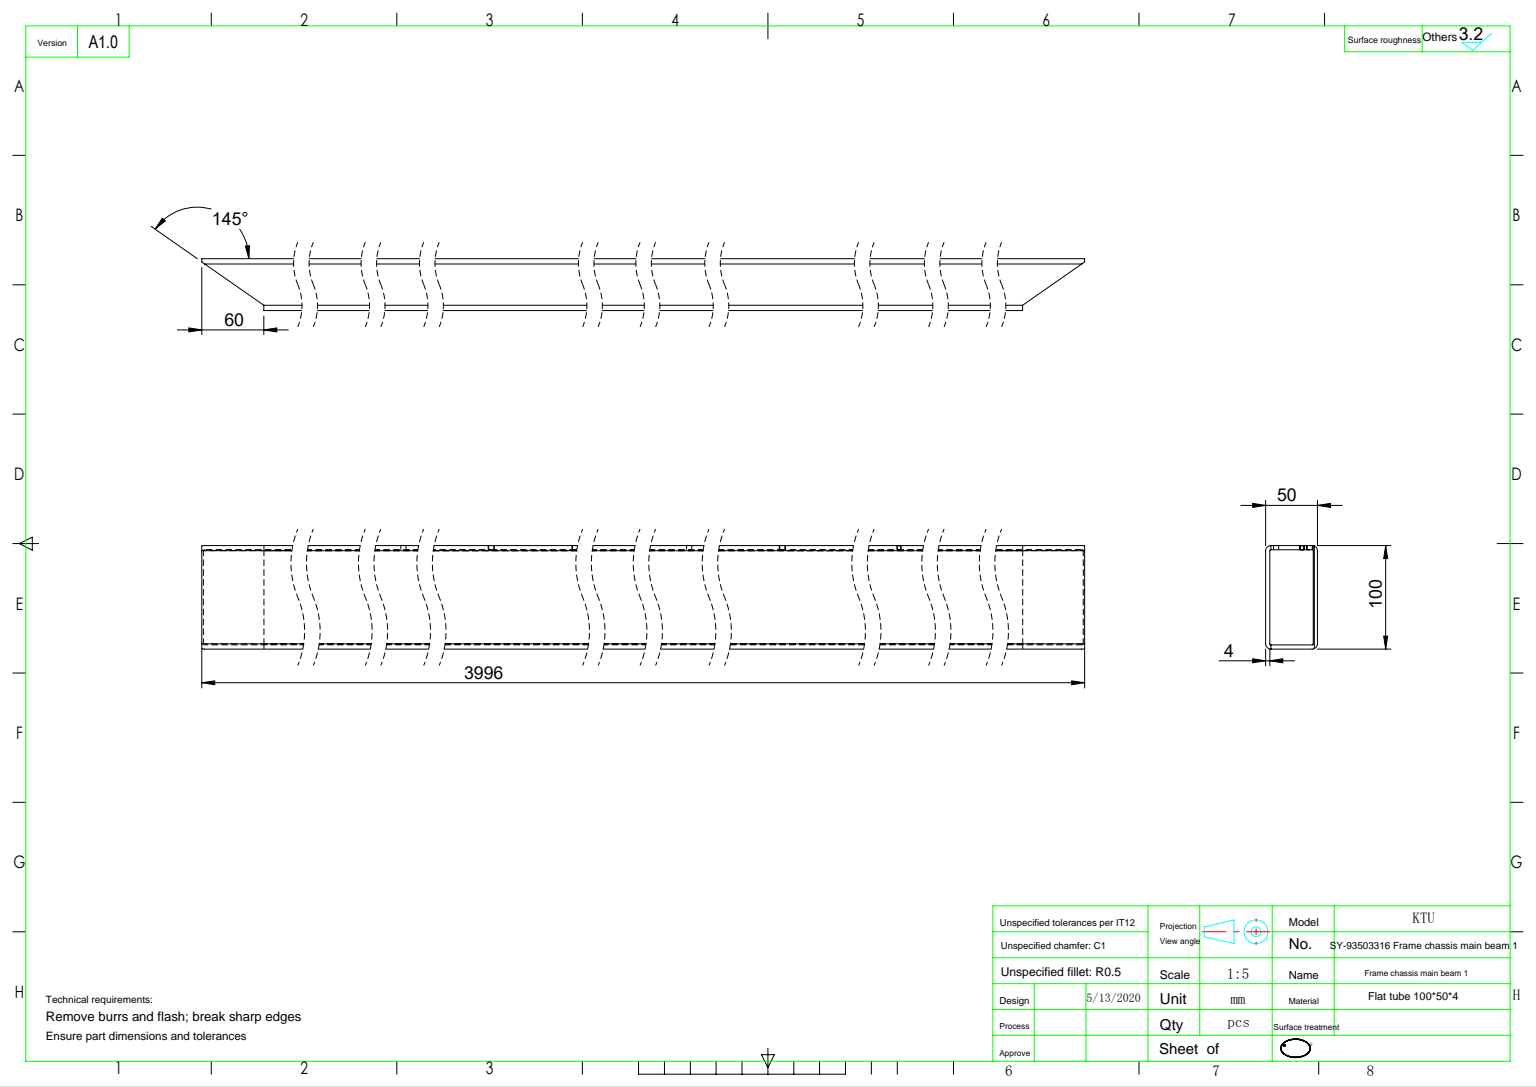
SolidWorks part; units mm, degrees
ref_plane "前视基准面" through (0, 0, 0) normal (0, 0, 1) x (1, 0, 0)
ref_plane "上视基准面" through (0, 0, 0) normal (0, 1, 0) x (1, 0, 0)
ref_plane "右视基准面" through (0, 0, 0) normal (1, 0, 0) x (0, 0, -1)
sketch "草图1" plane through (0, 0, 0) normal (0, 0, 1) x (1, 0, 0)
  line L1 (-20, 50) -> (20, 50)
  line L2 (-25, 45) -> (-25, -45)
  line L3 (-20, -50) -> (20, -50)
  line L4 (25, 45) -> (25, -45)
  line L5 (-25, 50) -> (25, -50) construction
  line L6 (-25, -50) -> (25, 50) construction
  arc A0 (20, -50) -> (25, -45) centre (20, -45) ccw
  arc A1 (-25, -45) -> (-20, -50) centre (-20, -45) ccw
  arc A2 (20, 50) -> (25, 45) centre (20, 45) cw
  arc A3 (-20, 50) -> (-25, 45) centre (-20, 45) ccw
  point P0 (0, 0)
  dimension "D3" = 5
  dimension "D1" = 50
  dimension "D2" = 100
extrude "拉伸-薄壁1" add sketch "草图1" along normal mid plane 3876 thin
sketch "草图7" plane through (0, 0, 1938) normal (0, 0, 1) x (1, 0, 0)
  line L0 (21, -45) -> (21, 45) construction
  line L1 (-20, -46) -> (20, -46) construction
  line L2 (-21, 45) -> (-21, -45) construction
  line L3 (20, 46) -> (-20, 46) construction
  line L4 (25, -45) -> (25, 45) construction
  line L5 (-20, -50) -> (20, -50) construction
  line L6 (-25, 45) -> (-25, -45) construction
  line L7 (20, 50) -> (-20, 50) construction
  line L8 (21, -45) -> (21, 45)
  line L9 (-20, -46) -> (20, -46)
  line L10 (-21, 45) -> (-21, -45)
  line L11 (20, 46) -> (-20, 46)
  line L12 (25, -45) -> (25, 45)
  line L13 (-20, -50) -> (20, -50)
  line L14 (-25, 45) -> (-25, -45)
  line L15 (20, 50) -> (-20, 50)
  arc A0 (21, 45) -> (20, 46) centre (20, 45) ccw construction
  arc A1 (-20, 46) -> (-21, 45) centre (-20, 45) ccw construction
  arc A2 (-21, -45) -> (-20, -46) centre (-20, -45) ccw construction
  arc A3 (20, -46) -> (21, -45) centre (20, -45) ccw construction
  arc A4 (25, 45) -> (20, 50) centre (20, 45) ccw construction
  arc A5 (20, -50) -> (25, -45) centre (20, -45) ccw construction
  arc A6 (-25, -45) -> (-20, -50) centre (-20, -45) ccw construction
  arc A7 (-20, 50) -> (-25, 45) centre (-20, 45) ccw construction
  arc A8 (21, 45) -> (20, 46) centre (20, 45) ccw
  arc A9 (-20, 46) -> (-21, 45) centre (-20, 45) ccw
  arc A10 (-21, -45) -> (-20, -46) centre (-20, -45) ccw
  arc A11 (20, -46) -> (21, -45) centre (20, -45) ccw
  arc A12 (25, 45) -> (20, 50) centre (20, 45) ccw
  arc A13 (20, -50) -> (25, -45) centre (20, -45) ccw
  arc A14 (-25, -45) -> (-20, -50) centre (-20, -45) ccw
  arc A15 (-20, 50) -> (-25, 45) centre (-20, 45) ccw
extrude "凸台-拉伸1" add sketch "草图7" along normal blind 60 separate body
sketch "草图8" plane through (0, 50, 0) normal (0, 1, 0) x (1, 0, 0)
  line L0 (20, -1938) -> (-22.0125, -1998)
  line L2 (20, -1998) -> (-20, -1998) construction
  line L3 (-22.0125, -1998) -> (31.9138, -1998)
  line L4 (31.9138, -1998) -> (31.9138, -1938)
  line L5 (31.9138, -1938) -> (20, -1938)
  line L6 (20, -1938) -> (-20, -1938) construction
  line L7 (0, 0) -> (86.3512, 0) construction
  dimension "D1" = 55
extrude "切除-拉伸2" cut sketch "草图8" against normal through all
ref_plane "基准面1" through (0, 0, 0) normal (0, 0, 1) x (1, 0, 0)
sketch "草图9" plane through (0, 0, -1938) normal (0, 0, -1) x (-1, 0, 0)
  line L0 (-20, 46) -> (20, 46) construction
  line L1 (-21, -45) -> (-21, 45) construction
  line L2 (20, -46) -> (-20, -46) construction
  line L3 (20, -50) -> (-20, -50) construction
  line L4 (-25, -45) -> (-25, 45) construction
  line L5 (21, 45) -> (21, -45) construction
  line L6 (25, 45) -> (25, -45) construction
  line L7 (-20, 50) -> (20, 50) construction
  line L8 (-20, 46) -> (20, 46)
  line L9 (-21, -45) -> (-21, 45)
  line L10 (20, -46) -> (-20, -46)
  line L11 (20, -50) -> (-20, -50)
  line L12 (-25, -45) -> (-25, 45)
  line L13 (21, 45) -> (21, -45)
  line L14 (25, 45) -> (25, -45)
  line L15 (-20, 50) -> (20, 50)
  arc A0 (-20, 46) -> (-21, 45) centre (-20, 45) ccw construction
  arc A1 (21, 45) -> (20, 46) centre (20, 45) ccw construction
  arc A2 (20, -46) -> (21, -45) centre (20, -45) ccw construction
  arc A3 (-21, -45) -> (-20, -46) centre (-20, -45) ccw construction
  arc A4 (-25, -45) -> (-20, -50) centre (-20, -45) ccw construction
  arc A5 (20, -50) -> (25, -45) centre (20, -45) ccw construction
  arc A6 (-20, 50) -> (-25, 45) centre (-20, 45) ccw construction
  arc A7 (25, 45) -> (20, 50) centre (20, 45) ccw construction
  arc A8 (-20, 46) -> (-21, 45) centre (-20, 45) ccw
  arc A9 (21, 45) -> (20, 46) centre (20, 45) ccw
  arc A10 (20, -46) -> (21, -45) centre (20, -45) ccw
  arc A11 (-21, -45) -> (-20, -46) centre (-20, -45) ccw
  arc A12 (-25, -45) -> (-20, -50) centre (-20, -45) ccw
  arc A13 (20, -50) -> (25, -45) centre (20, -45) ccw
  arc A14 (-20, 50) -> (-25, 45) centre (-20, 45) ccw
  arc A15 (25, 45) -> (20, 50) centre (20, 45) ccw
extrude "凸台-拉伸2" add sketch "草图9" along normal blind 60 separate body
sketch "草图10" plane through (0, 50, 0) normal (0, 1, 0) x (1, 0, 0)
  line L0 (20, 1938) -> (-22.0125, 1998)
  line L1 (-20, 1938) -> (20, 1938) construction
  line L2 (25, 1998) -> (25, 1938)
  line L3 (25, 1938) -> (20, 1938)
  line L4 (25, 1998) -> (-22.0125, 1998)
  dimension "D1" = 55
extrude "切除-拉伸3" cut sketch "草图10" against normal through all
hole_wizard "M6 螺纹孔1" positions "草图11" profile "草图12" tap size "M6" standard "GB"
sketch "草图11" plane through (0, 50, 0) normal (0, 1, 0) x (1, 0, 0)
  line L0 (-17.5, -543.5) -> (-17.5, -624.5) construction
  line L2 (-17.5, 624.5) -> (-17.5, 543.5) construction
  line L4 (-25, -1938) -> (-25, 1938) construction
  line L5 (-27.5, 0) -> (27.5, 0) construction
  point P0 (-17.5, 624.5)
  point P3 (-17.5, 543.5)
  point P6 (-17.5, -543.5)
  point P9 (-17.5, -624.5)
  dimension "D1" = 7.5
  dimension "D2" = 81
  dimension "D3" = 81
  dimension "D4" = 7.5
  dimension "D5" = 1087
  dimension "D6" = 624.5
sketch "草图12" plane through (-17.5, 50, -624.5) normal (1, 0, 0) x (0, 0, 1)
  line L0 (0, 0) -> (0, 16.5022)
  line L1 (0, 16.5022) -> (2.5, 15)
  line L2 (2.5, 15) -> (2.5, 0)
  line L5 (2.5, 0) -> (0, 0)
  line L10 (0, 16.5022) -> (-2.5, 15) construction
  line L11 (0, -6.35) -> (0, 107.95) construction
  dimension "螺纹孔钻头直径" = 5
  dimension "螺纹孔钻头深度" = 15
  dimension "导头角度" = 118
cosmetic thread "孔螺蚊线1" parameters "D1"=4, "D2"=6
cosmetic thread "孔螺蚊线2" parameters "D1"=4, "D2"=6
cosmetic thread "孔螺蚊线3" parameters "D1"=4, "D2"=6
cosmetic thread "孔螺蚊线4" parameters "D1"=4, "D2"=6
hole_wizard "大小mm 暗销孔1" positions "草图15" profile "草图14" hole size "Ø5.0" standard "GB"
sketch "草图15" plane through (0, 50, 0) normal (0, 1, 0) x (1, 0, 0)
  line L1 (11, 1518) -> (19, 1518) construction
  line L2 (11, 1522) -> (11, 1514) construction
  line L3 (19, 1514) -> (19, 1522) construction
  line L5 (11, 818) -> (19, 818) construction
  line L6 (11, 822) -> (11, 814) construction
  line L7 (19, 814) -> (19, 822) construction
  point P21 (15, 1518)
  point P23 (15, 818)
sketch "草图14" plane through (15, 50, -818) normal (1, 0, 0) x (0, 0, 1)
  line L0 (0, 0) -> (0, 10.0022)
  line L1 (0, 10.0022) -> (2.5, 8.5)
  line L2 (2.5, 8.5) -> (2.5, 0.025)
  line L3 (2.5, 0.025) -> (2.525, 0)
  line L5 (2.525, 0) -> (0, 0)
  line L6 (-2.5, 0.025) -> (-2.525, 0) construction
  line L10 (0, 10.0022) -> (-2.5, 8.5) construction
  line L11 (0, -6.35) -> (0, 107.95) construction
  dimension "孔直径" = 5
  dimension "孔深度" = 8.5
  dimension "近端锥形沉头孔直径" = 5.05
  dimension "近端锥形沉头孔角度" = 90
  dimension "导头角度" = 118
pattern_linear "阵列(线性)1" count 3 spacing 1168 along (0, 0, 1) of "大小mm 暗销孔1"
hole_wizard "M4 螺纹孔1" positions "草图16" profile "草图17" tap size "M4" standard "GB"
sketch "草图16" plane through (0, 50, 0) normal (0, 1, 0) x (1, 0, 0)
  point P0 (-10, -1628)
  point P3 (-10, -1098)
  point P6 (-10, -1077.4937)
  point P9 (-10, -757)
  point P12 (-10, -203)
  point P15 (-10, -182)
  point P18 (-10, 158)
  point P21 (-10, 693)
sketch "草图17" plane through (-10, 50, 1628) normal (1, 0, 0) x (0, 0, 1)
  line L0 (0, 0) -> (0, 11.0914)
  line L1 (0, 11.0914) -> (1.65, 10.1)
  line L2 (1.65, 10.1) -> (1.65, 0.375)
  line L3 (1.65, 0.375) -> (2.025, 0)
  line L5 (2.025, 0) -> (0, 0)
  line L6 (-1.65, 0.375) -> (-2.025, 0) construction
  line L10 (0, 11.0914) -> (-1.65, 10.1) construction
  line L11 (0, -6.35) -> (0, 107.95) construction
  dimension "螺纹孔钻头直径" = 3.3
  dimension "螺纹孔钻头深度" = 10.1
  dimension "近端锥形沉头孔直径" = 4.05
  dimension "近端锥形沉头孔角度" = 90
  dimension "导头角度" = 118
cosmetic thread "孔螺蚊线5" parameters "D1"=4, "D2"=4
cosmetic thread "孔螺蚊线6" parameters "D1"=4, "D2"=4
cosmetic thread "孔螺蚊线7" parameters "D1"=4, "D2"=4
cosmetic thread "孔螺蚊线8" parameters "D1"=4, "D2"=4
cosmetic thread "孔螺蚊线9" parameters "D1"=4, "D2"=4
cosmetic thread "孔螺蚊线10" parameters "D1"=4, "D2"=4
cosmetic thread "孔螺蚊线11" parameters "D1"=4, "D2"=4
cosmetic thread "孔螺蚊线12" parameters "D1"=4, "D2"=4
hole_wizard "M4 螺纹孔2" positions "草图18" profile "草图19" tap size "M4" standard "GB"
sketch "草图18" plane through (0, 50, 0) normal (0, 1, 0) x (1, 0, 0)
  point P0 (-10, 1453)
sketch "草图19" plane through (-10, 50, -1453) normal (1, 0, 0) x (0, 0, 1)
  line L0 (0, 0) -> (0, 11.0914)
  line L1 (0, 11.0914) -> (1.65, 10.1)
  line L2 (1.65, 10.1) -> (1.65, 0.375)
  line L3 (1.65, 0.375) -> (2.025, 0)
  line L5 (2.025, 0) -> (0, 0)
  line L6 (-1.65, 0.375) -> (-2.025, 0) construction
  line L10 (0, 11.0914) -> (-1.65, 10.1) construction
  line L11 (0, -6.35) -> (0, 107.95) construction
  dimension "螺纹孔钻头直径" = 3.3
  dimension "螺纹孔钻头深度" = 10.1
  dimension "近端锥形沉头孔直径" = 4.05
  dimension "近端锥形沉头孔角度" = 90
  dimension "导头角度" = 118
cosmetic thread "孔螺蚊线13" parameters "D1"=4, "D2"=4
combine bodies "组合1" operation type add bodies to combine 107 112
combine bodies "组合2" operation type add bodies to combine 113 105
sketch "草图20" plane through (0, 50, 0) normal (0, 1, 0) x (1, 0, 0)
  line L0 (-25, 1998) -> (-25, -1998) construction
  line L1 (-22.0125, 1998) -> (-25, 1998) construction
  circle A0 centre (-10, 1710) radius 1.65
  dimension "D1" = 3.3
  dimension "D3" = 288
  dimension "D2" = 15
extrude "切除-拉伸4" cut sketch "草图20" against normal blind 10
cosmetic thread "装饰螺纹线1" parameters "D2"=4
